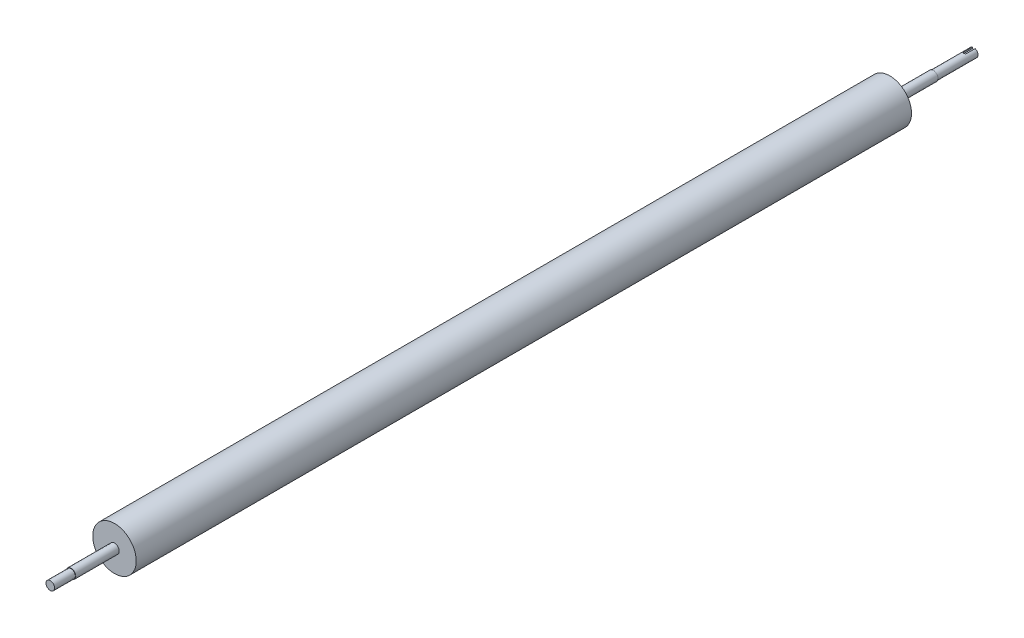
from build123d import *

# Parameters (mm, degrees)
SKETCH_1_R          = 38
EXTRUDE_1_DEPTH     = 678
SKETCH_2_R          = 7.5
EXTRUDE_2_DEPTH     = 146.75
SKETCH_3_R          = 8.25
EXTRUDE_4_DEPTH     = 76
EXTRUDE_START       = 76
SKETCH_4_R          = 8.25
EXTRUDE_5_DEPTH     = 76
CUT_EXTRUDE_START   = 7.5
CUT_EXTRUDE_2_DEPTH = 3
SKETCH_9_R          = 14.996083322
CUT_EXTRUDE_4_DEPTH = 34.45


with BuildPart() as part:
    # 草图1 → 凸台-拉伸1 (new, symmetric)
    with BuildSketch(Plane.XY):
        Circle(SKETCH_1_R)
    extrude(amount=EXTRUDE_1_DEPTH, both=True)

    # 草图2 → 凸台-拉伸2 (add, symmetric)
    with BuildSketch(Plane.XY.offset(678)):
        with Locations(Location((0, 0, 0), (0, 0, 180))):
            Circle(SKETCH_2_R)
    extrude_2 = extrude(amount=EXTRUDE_2_DEPTH, both=True)

    # 镜向1: 凸台-拉伸2 across plane
    add(extrude_2.mirror(Plane.XY))

    # 草图3 → 凸台-拉伸4 (add)
    with BuildSketch(Plane.XY.offset(678)):
        Circle(SKETCH_3_R)
    extrude(amount=EXTRUDE_4_DEPTH)

    # 草图4 → 凸台-拉伸5 (add)
    with BuildSketch(Plane(origin=(0, 0, -678), x_dir=(-1, 0, 0), z_dir=(0, 0, -1)).offset(EXTRUDE_START)):
        with Locations(Location((0, 0, 0), (0, 0, 180))):
            Circle(SKETCH_4_R)
    extrude(amount=-EXTRUDE_5_DEPTH)

    # 草图6 → 切除-拉伸2 (cut)
    with BuildSketch(Plane(origin=(0, 0, 0), x_dir=(1, 0, 0), z_dir=(0, 1, 0)).offset(CUT_EXTRUDE_START)):
        with BuildLine():
            Line((-2.5, -824.75), (-2.5, -809.75))
            ThreePointArc((-2.5, -809.75), (0, -807.25), (2.5, -809.75))
            Line((2.5, -809.75), (2.5, -824.75))
            ThreePointArc((2.5, -824.75), (0, -827.25), (-2.5, -824.75))
        make_face()
    cut_extrude_2 = extrude(amount=-CUT_EXTRUDE_2_DEPTH, mode=Mode.SUBTRACT)

    # 镜向2: 切除-拉伸2 across plane
    add(cut_extrude_2.mirror(Plane.XY), mode=Mode.SUBTRACT)

    # 草图9 → 切除-拉伸4 (cut)
    with BuildSketch(Plane.XY.offset(824.75)):
        Circle(SKETCH_9_R)
    extrude(amount=-CUT_EXTRUDE_4_DEPTH, mode=Mode.SUBTRACT)


solid = part.part
